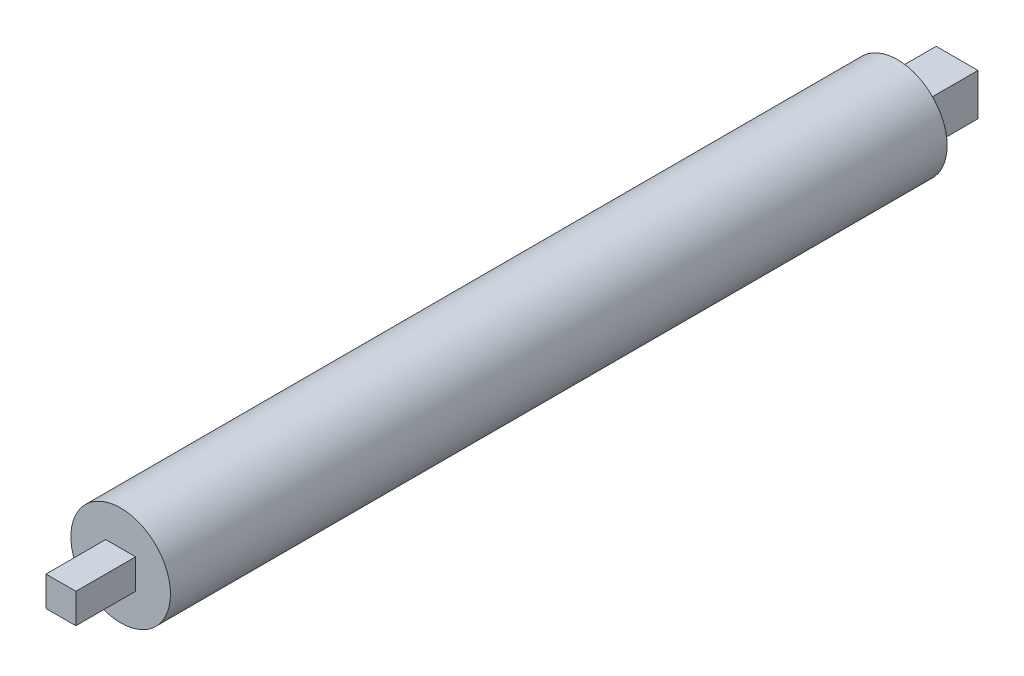
SolidWorks part; units mm, degrees
ref_plane "前视基准面" through (0, 0, 0) normal (0, 0, 1) x (1, 0, 0)
ref_plane "上视基准面" through (0, 0, 0) normal (0, 1, 0) x (1, 0, 0)
ref_plane "右视基准面" through (0, 0, 0) normal (1, 0, 0) x (0, 0, -1)
sketch "草图1" plane through (0, 0, 0) normal (0, 0, 1) x (1, 0, 0)
  circle A0 centre (0, 0) radius 25
  dimension "D1" = 50
extrude "凸台-拉伸1" add sketch "草图1" along normal mid plane 390
sketch "草图2" plane through (0, 0, 0) normal (0, 0, 1) x (1, 0, 0)
  line L1 (-7.5, 7.5) -> (7.5, 7.5)
  line L2 (-7.5, 7.5) -> (-7.5, -7.5)
  line L3 (-7.5, -7.5) -> (7.5, -7.5)
  line L4 (7.5, 7.5) -> (7.5, -7.5)
  line L5 (0, -7.5) -> (0, 7.5) construction
  line L6 (-7.5, 0) -> (7.5, 0) construction
  point P0 (0, 0)
  dimension "D1" = 15
extrude "凸台-拉伸2" add sketch "草图2" along normal mid plane 450
other "移动面1" face at (7.5, 0, -210) face at (0, -7.5, -210) face at (-7.5, 0, -210) face at (0, 7.5, -210) parameters "D1"=3
